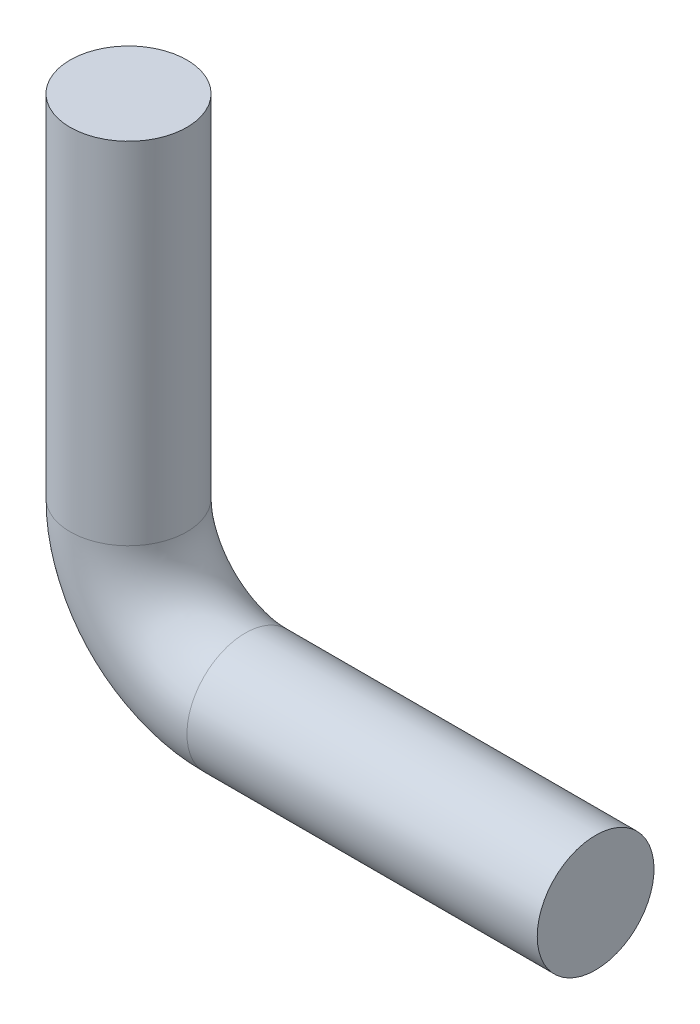
from build123d import *

# Parameters (mm, degrees)
SKETCH2_R = 6.35


with BuildPart() as part:
    # Sweep8: sweep along a path in Sketch1
    with BuildLine(Plane.XY) as sweep8_path:
        Line((-4.294322906, -24.238530735), (-42.394322906, -24.238530735))
        ThreePointArc((-42.394322906, -24.238530735), (-51.374579027, -20.518786856), (-55.094322906, -11.538530735))
        Line((-55.094322906, -11.538530735), (-55.094322906, 26.561469265))
    # Sketch2 → Sweep8 (sweep)
    with BuildSketch(Plane.ZY.offset(4.294322906)):
        with Locations((0, -24.238530735)):
            Circle(SKETCH2_R)
    sweep(path=sweep8_path.line)


solid = part.part
